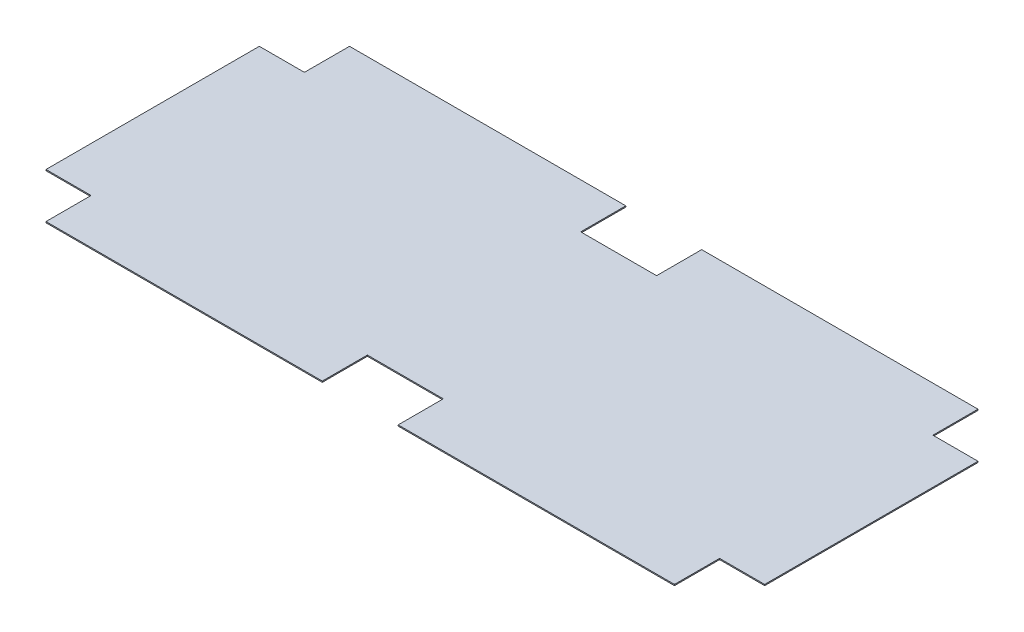
from build123d import *

# Parameters (mm, degrees)
BOSS_EXTRUDE_1_DEPTH = 8


with BuildPart() as part:
    # Sketch 1 → Boss-Extrude 1 (new body)
    with BuildSketch(Plane(origin=(0, 0, 0), x_dir=(1, 0, 0), z_dir=(0, 1, 0))):
        Polygon((2195, 1060), (265, 1060), (265, 745), (-265, 745), (-265, 1060), (-2195, 1060), (-2195, 745), (-2510, 745), (-2510, -745), (-2195, -745), (-2195, -1060), (-265, -1060), (-265, -745), (265, -745), (265, -1060), (2195, -1060), (2195, -745), (2510, -745), (2510, 745), (2195, 745), align=None)
    extrude(amount=BOSS_EXTRUDE_1_DEPTH)


solid = part.part
